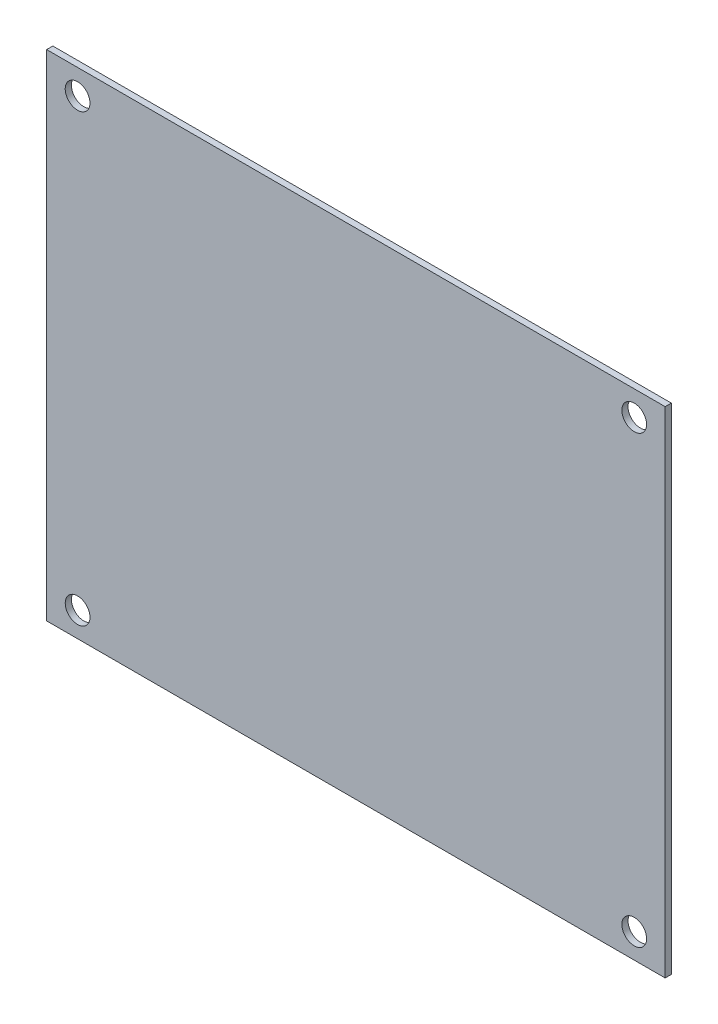
from build123d import *

# Parameters (mm, degrees)
SKETCH1_W           = 100
SKETCH1_H           = 80
SKETCH1_R           = 2
BOSS_EXTRUDE1_DEPTH = 1


with BuildPart() as part:
    # Sketch1 → Boss-Extrude1 (new body)
    with BuildSketch(Plane.XY):
        Rectangle(SKETCH1_W, SKETCH1_H)
        with Locations((45, 36)):
            Circle(SKETCH1_R, mode=Mode.SUBTRACT)
        with Locations((-45, 36)):
            Circle(SKETCH1_R, mode=Mode.SUBTRACT)
        with Locations(Location((-45, -36, 0), (0, 0, 180))):
            Circle(SKETCH1_R, mode=Mode.SUBTRACT)
        with Locations(Location((45, -36, 0), (0, 0, 180))):
            Circle(SKETCH1_R, mode=Mode.SUBTRACT)
    extrude(amount=BOSS_EXTRUDE1_DEPTH)


solid = part.part
